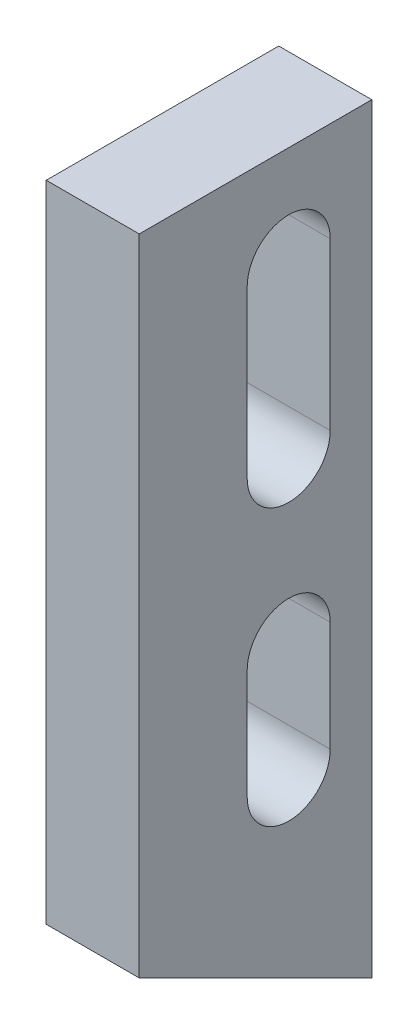
SolidWorks part; units mm, degrees
material "Q235-A"
ref_plane "Front Plane" through (0, 0, 0) normal (0, 0, 1) x (1, 0, 0)
ref_plane "Top Plane" through (0, 0, 0) normal (0, 1, 0) x (1, 0, 0)
ref_plane "Right Plane" through (0, 0, 0) normal (1, 0, 0) x (0, 0, -1)
sketch "Sketch1" plane through (0, 0, 0) normal (1, 0, 0) x (0, 0, -1)
  line L0 (0, 0) -> (70, -35)
  line L1 (70, -35) -> (70, 194)
  line L2 (70, 194) -> (0, 194)
  line L3 (0, 194) -> (0, 0)
  line L4 (45, 114) -> (45, 164) construction
  line L5 (32.5, 114) -> (32.5, 164)
  line L6 (57.5, 114) -> (57.5, 164)
  line L7 (45, 30.9103) -> (45, 64) construction
  line L8 (32.5, 30.9103) -> (32.5, 64)
  line L9 (57.5, 30.9103) -> (57.5, 64)
  arc A0 (32.5, 114) -> (57.5, 114) centre (45, 114) ccw
  arc A1 (57.5, 164) -> (32.5, 164) centre (45, 164) ccw
  arc A2 (32.5, 30.9103) -> (57.5, 30.9103) centre (45, 30.9103) ccw
  arc A3 (57.5, 64) -> (32.5, 64) centre (45, 64) ccw
  point P8 (45, 139)
  point P13 (45, 47.4552)
  dimension "D4" = 12.5
  dimension "D5" = 30
  dimension "D6" = 50
  dimension "D7" = 50
  dimension "D8" = 25
  dimension "D1" = 70
  dimension "D2" = 229
  dimension "D3" = 35
extrude "Boss-Extrude1" add sketch "Sketch1" along normal mid plane 40
chamfer "Chamfer1" distance 12 angle 45 4 edges at (-20, 79.5, -70) (-20, 194, -35) (-20, 97, 0) (-20, -17.5, -35)
